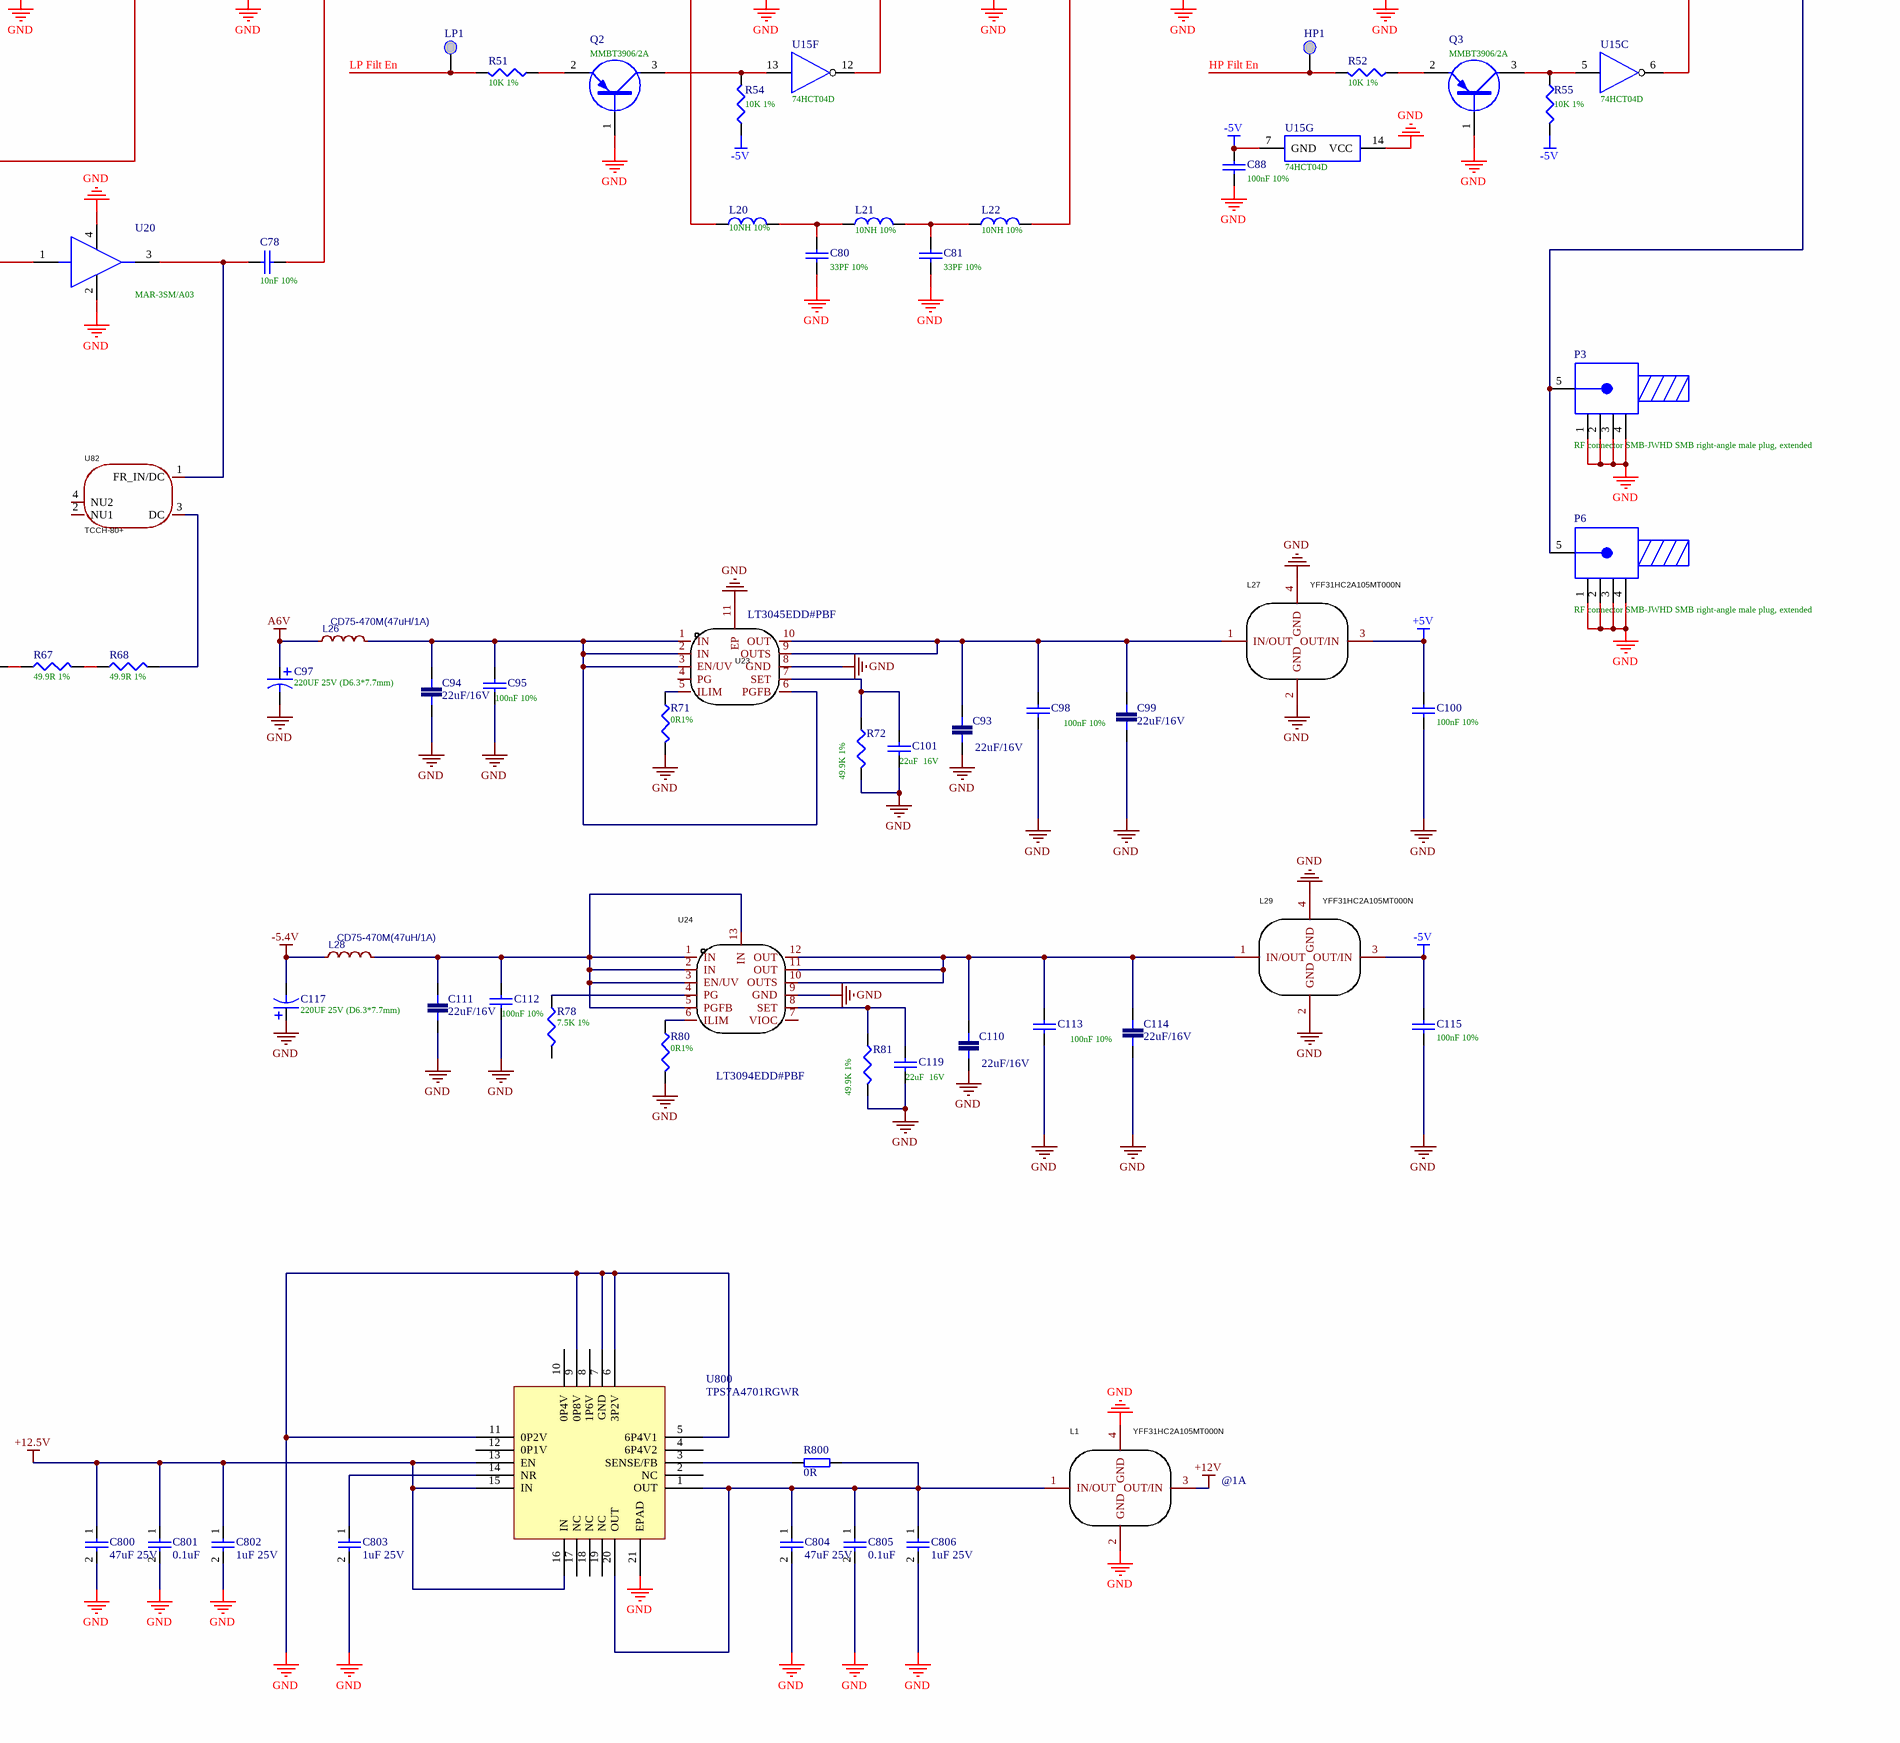
[diagram p0: PCBE109560-7.SchDoc, bottom right]
# Altium schematic sheet PCBE109560-7.SchDoc (part 2 of 2)

## Parts
1  (no value)  [DIP-1]
+1  (no value)  [DIP-1]
+2  (no value)  [DIP-1]
C4  20PF 10%  [0805C]
C5  330PF 10%  [1812C]
C6  22PF 10%  [1812C-2]
C7  22uF/16V  [0805]
C8  22uF/16V  [0805]
C9  100nF 10%  [0603]
C10  220UF 25V (D6.3*7.7mm)  [CAP-SMD_BD6.3-L6.6-W6.6-FD]
C11  100nF 10%  [0603]
C12  22uF/16V  [0805]
C13  100nF 10%  [0805R]
C14  22uF  16V  [0805]
C15  100nF 10%  [0805R]
C16  47PF 10%  [1812C-2]
C17  100PF 10%  [1812C-2]
C18  20PF 10%  [0805R]
C20  100nF 10%  [0805R]
C21  100nF 10%  [0805R]
C31  100nF 10%  [0805R]
C32  100nF 10%  [0805R]
C34  100nF 10%  [0805R]
C35  100nF 10%  [0805R]
C36  100nF 10%  [0805R]
C37  100nF 10%  [0805R]
C39  100nF 10%  [0805R]
C40  100nF 10%  [0805R]
C41  100nF 10%  [0805R]
C42  100nF 10%  [0805R]
C43  100nF 10%  [0805R]
C44  100nF 10%  [0805R]
C45  100nF 10%  [0805R]
C46  100nF 10%  [0805R]
C47  100nF 10%  [0805R]
C48  100nF 10%  [0805R]
C49  22uF 25V  [CAP-SMD_L6.0-W3.2-R-RD]
C50  100nF 10%  [0805R]
C51  100nF 10%  [0805R]
C52  100nF 10%  [0805R]
C53  3.3NF 10%  [0805R]
C54  100nF 10%  [0805R]
C55  330PF 10%  [0805R]
C56  330PF 10%  [0805R]
C57  100nF 10%  [0805R]
C58  33PF 10%  [0805R]
C59  33PF 10%  [0805R]
C60  100nF 10%  [0805R]
C61  100nF 10%  [0805R]
C62  100nF 10%  [0805R]
C63  100nF 10%  [0805R]
C64  100nF 10%  [0805R]
C65  33PF 10%  [0805R]
C66  33PF 10%  [0805R]
C67  100nF 10%  [0805R]
C68  39PF 10%  [0805R]
C69  100nF 10%  [0805R]
C70  25V 1UF Type A  [0805C-2]
C71  25V 1UF Type A  [0805C-2]
C72  100nF 10%  [0805R]
C73  25V 1UF Type A  [0805C-2]
C74  100nF 10%  [0805R]
C75  100nF 10%  [0805R]
C76  10nF 10%  [0805R]
C77  10nF 10%  [0805R]
C78  10nF 10%  [0805R]
C79  100nF 10%  [0603C]
C80  33PF 10%  [0805R]
C81  33PF 10%  [0805R]
C82  100nF 10%  [0805R]
C83  100nF 10%  [0805R]
C84  100nF 10%  [0805R]
C85  100nF 10%  [0805R]
C86  25V 1UF Type A  [0805C-2]
C87  3pF( ±0.1pF)  [0805R]
C88  100nF 10%  [0805R]
C89  100nF 10%  [0805R]
C90  100nF 10%  [0805R]
C93  22uF/16V  [0805]
C94  22uF/16V  [0805]
C95  100nF 10%  [0603]
C96  100nF 10%  [0805R]
C97  220UF 25V (D6.3*7.7mm)  [CAP-SMD_BD6.3-L6.6-W6.6-FD]
C98  100nF 10%  [0603]
C99  22uF/16V  [0805]
C100  100nF 10%  [0805R]
C101  22uF  16V  [0805]
C102  100nF 10%  [0805R]
C103  100nF 10%  [0805R]
C104  100nF 10%  [0805R]
C105  100nF 10%  [0805R]
C106  100nF 10%  [0805R]
C107  100nF 10%  [0805R]
C109  100nF 10%  [0805R]
C110  22uF/16V  [0805]
C111  22uF/16V  [0805]
C112  100nF 10%  [0603]
C113  100nF 10%  [0603]
C114  22uF/16V  [0805]
C115  100nF 10%  [0805R]
C116  100nF 10%  [0805R]
C117  220UF 25V (D6.3*7.7mm)  [CAP-SMD_BD6.3-L6.6-W6.6-FD]
C118  100nF 10%  [0805R]
C119  22uF  16V  [0805]
C122  100nF 10%  [0805R]
C123  100nF 10%  [0805R]
C124  100nF 10%  [0805R]
C125  100nF 10%  [0805R]
C128  100nF 10%  [0805R]
C129  100nF 10%  [0805R]
C130  100nF 10%  [0805R]
C800  47uF 25V  [1206]
C801  0.1uF  [0402]
C802  1uF 25V  [0402]
C803  1uF 25V  [0402]
C804  47uF 25V  [1206]
C805  0.1uF  [0402]
C806  1uF 25V  [0402]
C?  100nF 10%  [0805R]
Clk1  (no value)  [DIP-1]
D1  BAV99/A7  [SOT-23]
D2  GF1M-E3/67A/GM  [1808D]
D3  GF1M-E3/67A/GM  [1808D]
D4  GF1M-E3/67A/GM  [1808D]
D5  GF1M-E3/67A/GM  [1808D]
D8  BAV99/A7  [SOT-23-2]
D9  BAV99/A7  [SOT-23-2]
D10  BAV99/A7  [SOT-23-2]
D11  BAV99/A7  [SOT-23-2]
D12  BAV99/A7  [SOT-23-2]
Data1  (no value)  [DIP-1]
HP1  (no value)  [DIP-1]
J1  RF connector  [DIP-P]
J2  RF connector  [DIP-P]
L1  YFF31HC2A105MT000N  [FILTER-SMD_4P-L3.2-W1.6-L_YFF31HC]
L2  15UH 5%  [1005R]
L3  BLM21PG221SN1D(220Ω@100MHz)  [0805R]
L4  YFF31HC2A105MT000N  [FILTER-SMD_4P-L3.2-W1.6-L_YFF31HC]
L5  6.8UH 10%  [0805R]
L8  YFF31HC2A105MT000N  [FILTER-SMD_4P-L3.2-W1.6-L_YFF31HC]
L10  10NH 10%  [0805R]
L11  10NH 10%  [0805R]
L12  10NH 10%  [0805R]
L13  YFF31HC2A105MT000N  [FILTER-SMD_4P-L3.2-W1.6-L_YFF31HC]
L15  4.7UH 5%  [1005L]
L16  1UH 5%  [0805R]
L17  BLM21PG221SN1D(220Ω@100MHz)  [0805R]
L18  BLM21PG221SN1D(220Ω@100MHz  [0805R]
L19  NFM15PC104R1A3D  [FILTER-SMD_0402-3P-L1.0-W0.5-T]
L20  10NH 10%  [0805R]
L21  10NH 10%  [0805R]
L22  10NH 10%  [0805R]
L23  YFF31HC2A105MT000N  [FILTER-SMD_4P-L3.2-W1.6-L_YFF31HC]
L24  YFF31HC2A105MT000N  [FILTER-SMD_4P-L3.2-W1.6-L_YFF31HC]
L25  BLM21PG221SN1D(220Ω@100MHz  [0805R]
L26  CD75-470M(47uH/1A)  [IND-SMD_L7.8-W7.0-A]
L27  YFF31HC2A105MT000N  [FILTER-SMD_4P-L3.2-W1.6-L_YFF31HC]
L28  CD75-470M(47uH/1A)  [IND-SMD_L7.8-W7.0-A]
L29  YFF31HC2A105MT000N  [FILTER-SMD_4P-L3.2-W1.6-L_YFF31HC]
L31  BLM21PG221SN1D(220Ω@100MHz  [0805R]
L32  BLM21PG221SN1D(220Ω@100MHz  [0805R]
L808  NFM15PC104R1A3D  [FILTER-SMD_0402-3P-L1.0-W0.5-T]
L809  NFM15PC104R1A3D  [FILTER-SMD_0402-3P-L1.0-W0.5-T]
L810  NFM15PC104R1A3D  [FILTER-SMD_0402-3P-L1.0-W0.5-T]
L811  NFM15PC104R1A3D  [FILTER-SMD_0402-3P-L1.0-W0.5-T]
L812  NFM15PC104R1A3D  [FILTER-SMD_0402-3P-L1.0-W0.5-T]
L813  NFM15PC104R1A3D  [FILTER-SMD_0402-3P-L1.0-W0.5-T]
LP1  (no value)  [DIP-1]
P1  Header 20X2  [N0.8mm/40Pin-Plug]
P2  Header 4X2  [N0.8mm/8Pin-SOCKET]
P3  RF connector SMB-JWHD SMB right-angle male plug, extended  [DIP-P-2]
P4  Header 20X2  [N0.8mm/40Pin-Plug]
P5  Header 20X2  [N0.8mm/40Pin-Plug]
P6  RF connector SMB-JWHD SMB right-angle male plug, extended  [DIP-P-2]
Q1  MJD31C  [SOT-252-2]
Q2  MMBT3906/2A  [SOT-23]
Q3  MMBT3906/2A  [SOT-23]
Q4  MMBT3906/2A  [SOT-23]
R6  2K 5%  [0603R]
R7  NC  [AXIAL-0.51]
R8  3.9K 5% 1/2W  [AXIAL-0.51]
R9  3.9K 5% 1/2W  [AXIAL-0.51]
R10  3.9K 5% 1/2W  [AXIAL-0.51]
R11  3.9K 5% 1/2W  [AXIAL-0.51]
R13  0R1%  [0603]
R14  49.9K 1%  [0603]
R15  4.99K 1%  [0805R]
R16  2K 1%  [0805R]
R17  49.9R 1% 1/4W  [AXIAL-0.4]
R20  100R 1% 1/4W  [AXIAL-0.4]
R23  100R 1% 1/4W  [AXIAL-0.4]
R27  4.87K 1%  [0805R]
R28  4.87K 1%  [0805R]
R29  4.87K 1%  [0805R]
R30  4.87K 1%  [0805R]
R31  4.87K 1%  [0805R]
R32  10K 1%  [0805R]
R33  100K 1%  [0805R]
R34  100K 1%  [0805R]
R35  49.9R 1%  [0805R]
R36  49.9R 1%  [0805R]
R37  49.9R 1%  [0805R]
R38  49.9R 1%  [0805R]
R39  49.9R 1%  [0805R]
R40  49.9R 1% 1/4W  [R-SMD_L3.5-W1.5]
R41  10K 1%  [0805R]
R42  4.87K 1%  [0805R]
R43  4.87K 1%  [0805R]
R44  4.87K 1%  [0805R]
R45  4.87K 1%  [0805R]
R46  169R 1%  [0805R]
R47  169R 1%  [0805R]
R48  169R 1%  [0805R]
R49  49.9R 1%  [0805R]
R50  49.9R 1%  [0805R]
R51  10K 1%  [0805R]
R52  10K 1%  [0805R]
R53  10K 1%  [0805R]
R54  10K 1%  [0805R]
R55  10K 1%  [0805R]
R56  10K 1%  [0805R]
R57  10K 1%  [0805R]
R58  49.9R 1%  [0805R]
R59  4.99K 1%  [0805R]
R60  49.9R 1%  [R-SMD_L3.5-W1.5]
R61  30R 1%  [R-SMD_L3.5-W1.5]
R62  169R 1%  [0805R]
R63  169R 1%  [0805R]
R64  169R 1%  [0805R]
R65  49.9R 1%  [0805R]
R66  49.9R 1%  [0805R]
R67  49.9R 1%  [0805R]
R68  49.9R 1%  [0805R]
R69  120R 1%  [R-SMD_L3.5-W1.5]
R70  169R 1%  [0805R]
R71  0R1%  [0603]
R72  49.9K 1%  [0603]
R73  169R 1%  [0805R]
R74  NC  [0805R]
R75  169R 1%  [0805R]
R77  169R 1%  [0805R]
R78  7.5K 1%  [0603]
R80  0R1%  [0603]
R81  49.9K 1%  [0603]
R82  100K 1%  [0805R]
R83  10K 1%  [0805R]
R84  169R 1%  [0805R]
R800  0R  [0402]
RE1  AGQ210A4HZ  [RELAY-SMD_PANASONIC_AGQ2X0AXX]
RE2  AGQ210A4HZ  [RELAY-SMD_PANASONIC_AGQ2X0AXX]
RE3  AGQ210A4HZ  [RELAY-SMD_PANASONIC_AGQ2X0AXX]
RE4  AGQ210A4HZ  [RELAY-SMD_PANASONIC_AGQ2X0AXX]
RE5  AGQ210A4HZ  [RELAY-SMD_PANASONIC_AGQ2X0AXX]
Strobe1  (no value)  [DIP-1]
U4  LT3045EDD#PBF  [DFN-10_L3.0-W3.0-P0.50-BL-EP]
U6  74HCT123D  [SOIC-16_L9.9-W3.9-P1.27-LS6.0-BL]
U8  MAX504CSD+T  [SO-14]
U9  SW-239  [SO-8]
U11  SW-239  [SO-8]
U12  SW-239  [SO-8]
U13  SW-239  [SO-8]
U14  SW-239  [SO-8]
U15  74HCT04D  [SO-14]  (parts A,B,C,D,E,F,G of 7)
U16  AT-250(MAAV-007941)  [SO-8]
U17  MAR-3SM/A03  [LCC4]
U18  MAR-6SM/A06  [LCC4]
U19  MAR-6SM/A06  [LCC4]
U20  MAR-3SM/A03  [LCC4]
U21  MAX4106ESA+T  [SO-8]
U22  MIC4420CM  [SO-8]
U23  LT3045EDD#PBF  [DFN-10_L3.0-W3.0-P0.50-BL-EP]
U24  LT3094EDD#PBF  [WDFN-12_L3.0-W3.0-P0.45-BL-EP]
U25  AT65-0263  [SO-16]
U80  TCCH-80+  [IND-SMD_4P-L3.8-W3.8]
U81  TCCH-80+  [IND-SMD_4P-L3.8-W3.8]
U82  TCCH-80+  [IND-SMD_4P-L3.8-W3.8]
U83  TCCH-80+  [IND-SMD_4P-L3.8-W3.8]
U100  SW-239  [SO-8]
U800  TPS7A4701RGWR  [QFN-20]

## Nets
+5V: C100.1 C?.1 L25.1 L27.3(OUT/IN) L811.3(OUTPUT) L812.3(OUTPUT) U8.3(~{CLR})
+12.5V: +2.1 C106.1 C800.1 C801.1 C802.1 P5.31 P5.32 P5.33 P5.34 P5.35 P5.36 P5.37 P5.38 P5.39 P5.40 U800.13(EN) U800.15(IN) U800.16(IN)
+12V: C122.1 C123.1 C124.2 C125.2 L1.3(OUT/IN) L8.1(IN/OUT) L13.1(IN/OUT) U22.1(VS) U22.8(VS)
-5.4V: +1.1 C107.1 C117.2 L28.2 P5.1 P5.2 P5.3 P5.4 P5.5 P5.6 P5.7 P5.8 P5.9 P5.10
-5V: C88.2 C115.2 L29.3(OUT/IN) L809.1(INPUT) L810.3(OUTPUT) L813.3(OUTPUT) R54.1 R55.2 R57.1 U15.7(GND)
A6V: 1.1 C10.1 C97.1 C103.2 L3.1 L26.2 P5.17 P5.18 P5.19 P5.20 P5.21 P5.22 P5.23 P5.24
GND: C5.1 C6.2 C7.1 C8.1 C9.2 C10.2 C11.2 C12.1 C13.2 C14.2 C15.1 C18.2 C20.1 C21.1 C31.1 C32.1 C34.1 C35.1 C36.2 C37.2 C39.2 C40.2 C42.2 C43.1 C44.2 C45.2 C46.2 C47.1 C48.1 C49.2 C50.2 C57.2 C60.2 C61.1 C62.1 C63.1 C64.1 C65.2 C66.1 C70.1 C71.1 C72.2 C73.1 C74.1 C75.1 C80.1 C81.1 C83.2 C84.2 C85.1 C86.2 C88.1 C89.2 C90.2 C93.1 C94.1 C95.2 C96.2 C97.2 C98.2 C99.1 C100.2 C101.2 C102.2 C103.1 C104.2 C105.1 C106.2 C107.2 C109.2 C110.1 C111.1 C112.2 C113.2 C114.1 C115.1 C117.1 C118.2 C119.2 C122.2 C123.2 C124.1 C125.1 C128.1 C129.1 C130.2 C800.2 C801.2 C802.2 C803.2 C804.2 C805.2 C806.2 C?.2 D1.3 D2.2(K) D11.2 D12.1 J1.1 J1.2 J1.3 J1.4 J2.1 J2.2 J2.3 J2.4 L1.2(GND) L1.4(GND) L2.2 L4.2(GND) L4.4(GND) L8.2(GND) L8.4(GND) L13.2(GND) L13.4(GND) L15.2 L16.1 L19.2(GND) L23.2(GND) L23.4(GND) L24.2(GND) L24.4(GND) L27.2(GND) L27.4(GND) L29.2(GND) L29.4(GND) L808.2(GND) L809.2(GND) L810.2(GND) L811.2(GND) L812.2(GND) L813.2(GND) P1.5 P1.6 P1.11 P1.12 P1.17 P1.18 P1.20 P1.23 P1.24 P1.29 P1.30 P1.35 P1.36 P2.1 P2.3 P2.5 P2.7 P3.1 P3.2 P3.3 P3.4 P4.5 P4.6 P4.11 P4.12 P4.17 P4.18 P4.23 P4.24 P4.29 P4.30 P4.35 P4.36 P5.11 P5.12 P5.13 P5.14 P5.15 P5.16 P5.25 P5.26 P5.27 P5.28 P5.29 P5.30 P6.1 P6.2 P6.3 P6.4 Q1.2(E) Q2.1(B) Q3.1(B) Q4.1(B) R13.2 R14.2 R20.2 R32.2 R53.1 R59.1 R61.1 R71.2 R72.2 R74.1 R80.2 R81.2 R82.1 R83.1 RE1.3 RE3.6 RE4.2 U4.8(GND) U4.11(EP) U6.6(2CEXT) U6.8(GND) U6.10(2B) U6.14(1CEXT) U8.7(DGND) U8.8(AGND) U9.2(GND) U9.7(GND) U9.8(GND) U11.2(GND) U11.7(GND) U11.8(GND) U12.2(GND) U12.7(GND) U12.8(GND) U13.2(GND) U13.7(GND) U13.8(GND) U14.2(GND) U14.7(GND) U14.8(GND) U15.14(VCC) U16.2(GND) U16.3(GND) U16.5(GND) U16.6(GND) U16.7(GND) U17.2(GND) U17.4(GND) U18.2(GND) U18.4(GND) U19.2(GND) U19.4(GND) U20.2(GND) U20.4(GND) U22.4(GND) U22.5(GND) U23.8(GND) U23.11(EP) U24.9(GND) U25.2(GND) U25.3(GND) U25.4(GND) U25.5(GND) U25.6(GND) U25.7(GND) U25.16(GND) U100.2(GND) U100.7(GND) U100.8(GND) U800.5(6P4V1) U800.6(3P2V) U800.7(GND) U800.9(0P8V) U800.11(0P2V) U800.21(EPAD)
VCC: C13.1 C15.2 L4.3(OUT/IN) R15.1 R16.2 U6.2(1B) U6.3(1~{R}D) U6.16(VCC)
AK2: C21.2 P1.33 RE1.1
AK3: C20.2 P1.38 RE1.8
AK4: C37.1 P1.37 RE2.1
AK5: C36.1 P1.40 RE2.8
AK6: C31.2 P1.34 RE3.8
AK7: C32.2 P1.32 RE3.1
AK8: C34.2 C40.1 P1.28 RE4.8 RE5.8
AK9: C35.2 C39.1 P1.26 RE4.1 RE5.1
Attn1: P4.34 R70.2
Attn2: P4.32 R73.2
Attn4: P4.28 R75.2
Attn8: P4.26 R77.2
Attn16: P4.22 R84.2
DAC Clk: Clk1.1 P4.14 U8.4(SCLK)
DAC Data: Data1.1 P4.16 U8.2(DIN)
DAC Strobe: P4.10 Strobe1.1 U8.5(~{CS})
DATA_T: P1.39 R15.2 U6.1(1~{A})
HP Filt En: HP1.1 P4.4 R52.2
HT: L5.1 P2.2 P2.4 P2.6 P2.8
IN2: P4.8 R56.1 U22.2(IN)
LP Filt En: LP1.1 P4.2 R51.2
NetC4_1: C4.1 D1.2 L2.1 Q1.1(B) R6.1
NetC4_2: C4.2 R6.2 U6.13(1Q)
NetC5_2: C5.2 L5.2 R7.2
NetC6_1: C6.1 C16.2 C17.2 Q1.3(C) R11.1
NetC7_2: C7.2 C11.1 C12.2 L4.1(IN/OUT) U4.9(OUTS) U4.10(OUT)
NetC8_2: C8.2 C9.1 L3.2 U4.1(IN) U4.2(IN) U4.3(EN/UV) U4.6(PGFB)
NetC14_1: C14.1 R14.1 U4.7(SET)
NetC16_1: C16.1 D5.1(A) D8.2 D9.2 RE2.6
NetC17_1: C17.1 RE2.7
NetC18_1: C18.1 R16.1 U6.15(1REXT/CEXT)
NetC41_1: C41.1 U14.1(RFCOM)
NetC41_2: C41.2 P3.5 P6.5 R32.1
NetC42_1: C42.1 R27.1 U9.5(B)
NetC43_2: C43.2 R28.2 U100.4(A)
NetC44_1: C44.1 R29.1 U11.4(A)
NetC45_1: C45.1 R30.1 U12.5(B)
NetC46_1: C46.1 R31.1 U13.5(B) U14.4(A)
NetC47_2: C47.2 R35.1 U16.4(A)
NetC48_2: C48.2 L8.3(OUT/IN) R36.1
NetC49_1: C49.1 C50.1 U8.1(BIPOFF) U8.9(REFIN) U8.10(REFOUT)
NetC51_1: C51.1 U17.1(RF_IN)
NetC51_2: C51.2 U16.8(RF2)
NetC52_1: C52.1 L10.2
NetC52_2: C52.2 U17.3(RF_OUT) U81.1(FR_IN/DC)
NetC53_1: C53.1 C54.1 L15.1
NetC53_2: C53.2 U12.1(RFCOM)
NetC54_2: C54.2 U13.1(RFCOM)
NetC55_1: C55.1 U13.3(RF1)
NetC55_2: C55.2 C56.1 L16.2
NetC56_2: C56.2 U14.6(RF2)
NetC57_1: C57.1 R41.1 U13.4(A) U14.5(B)
NetC58_1: C58.1 C65.1
NetC58_2: C58.2 L10.1 L11.1
NetC59_1: C59.1 L11.2 L12.1
NetC59_2: C59.2 C66.2
NetC60_1: C60.1 R42.1 U9.4(A)
NetC61_2: C61.2 R43.2 U100.5(B)
NetC62_2: C62.2 R44.1 U11.5(B)
NetC63_2: C63.2 R45.1 U12.4(A)
NetC64_2: C64.2 L13.3(OUT/IN) R46.2
NetC67_1: C67.1 U18.1(RF_IN)
NetC67_2: C67.2 U25.1(RF)
NetC68_1: C68.1 C69.2 R49.2 R50.2
NetC68_2: C68.2 R49.1 R50.1 U18.3(RF_OUT) U80.1(FR_IN/DC)
NetC69_1: C69.1 R53.2 U16.1(RF1)
NetC70_2: C70.2 C74.2 L18.1 L19.1(INPUT)
NetC71_2: C71.2 C75.2 L19.3(OUTPUT) U21.4(VEE)
NetC72_1: C72.1 C73.2 L17.2 L18.2
NetC76_1: C76.1 U9.3(RF1)
NetC76_2: C76.2 U19.1(RF_IN)
NetC77_1: C77.1 U19.3(RF_OUT) U83.1(FR_IN/DC)
NetC77_2: C77.2 U20.1(RF_IN)
NetC78_1: C78.1 U20.3(RF_OUT) U82.1(FR_IN/DC)
NetC78_2: C78.2 U100.6(RF2)
NetC79_1: C79.1 D10.3 R40.2
NetC79_2: C79.2 R58.2 R59.2
NetC80_2: C80.2 L20.2 L21.2
NetC81_2: C81.2 L21.1 L22.1
NetC82_1: C82.1 R60.2
NetC82_2: C82.2 C116.1 R74.2 R82.2
NetC83_1: C83.1 C86.1 L808.1(INPUT) U21.7(VCC)
NetC84_1: C84.1 L23.3(OUT/IN) R62.2
NetC85_2: C85.2 L24.3(OUT/IN) R65.1
NetC87_1: C87.1 R60.1 R69.1 U21.6(OUT)
NetC87_2: C87.2 R61.2 R69.2 U21.2(IN-)
NetC89_1: C89.1 L813.1(INPUT) U8.11(VSS)
NetC90_1: C90.1 L32.2 L811.1(INPUT)
NetC93_2: C93.2 C98.1 C99.2 L27.1(IN/OUT) U23.9(OUTS) U23.10(OUT)
NetC94_2: C94.2 C95.1 L26.1 U23.1(IN) U23.2(IN) U23.3(EN/UV) U23.6(PGFB)
NetC96_1: C96.1 R70.1 U25.15(C1)
NetC101_1: C101.1 R72.1 U23.7(SET)
NetC102_1: C102.1 R73.1 U25.14(C2)
NetC104_1: C104.1 L812.1(INPUT) U8.13(VDD)
NetC105_2: C105.2 L31.1 L810.1(INPUT)
NetC109_1: C109.1 R75.1 U25.13(C4)
NetC110_2: C110.2 C113.1 C114.2 L29.1(IN/OUT) U24.10(OUTS) U24.11(OUT) U24.12(OUT)
NetC111_2: C111.2 C112.1 L28.1 U24.1(IN) U24.2(IN) U24.3(EN/UV) U24.5(PGFB) U24.13(IN)
NetC116_2: C116.2 R83.2 U25.8(RF)
NetC118_1: C118.1 R77.1 U25.12(C8)
NetC119_1: C119.1 R81.1 U24.8(SET)
NetC128_2: C128.2 L31.2 U25.11(VEE)
NetC129_2: C129.2 L32.1 U25.10(VCC)
NetC130_1: C130.1 R84.1 U25.9(C16)
NetC803_1: C803.1 U800.14(NR)
NetC804_1: C804.1 C805.1 C806.1 L1.1(IN/OUT) R800.1 U800.1(OUT) U800.20(OUT)
NetD2_1: D2.1(A) D3.2(K)
NetD3_1: D3.1(A) D4.2(K)
NetD4_1: D4.1(A) D5.2(K)
NetD8_1: D8.1 D9.1 J1.5 R17.1 R20.1 R23.1 RE4.4
NetD10_1: D10.1 D12.2
NetD10_2: D10.2 D11.1
NetJ2_5: J2.5 RE5.4
NetL12_2: L12.2 U9.1(RFCOM)
NetL17_1: L17.1 L809.3(OUTPUT)
NetL20_1: L20.1 U11.6(RF2)
NetL22_2: L22.2 U12.3(RF1)
NetL23_1: L23.1(IN/OUT) L24.1(IN/OUT) U22.6(OUT) U22.7(OUT)
NetL25_2: L25.2 L808.3(OUTPUT)
NetQ2_2: Q2.2(E) R51.1
NetQ2_3: Q2.3(C) R54.2 U15.13(6A)
NetQ3_2: Q3.2(E) R52.1
NetQ3_3: Q3.3(C) R55.1 U15.5(3A)
NetQ4_2: Q4.2(E) R56.2
NetQ4_3: Q4.3(C) R57.2 U15.1(1A)
NetR7_1: R7.1 R8.1
NetR8_2: R8.2 R9.2
NetR9_1: R9.1 R10.1
NetR10_2: R10.2 R11.2
NetR13_1: R13.1 U4.5(ILIM)
NetR17_2: R17.2 RE1.2
NetR23_2: R23.2 RE3.7
NetR27_2: R27.2 R28.1 U15.4(2Y)
NetR29_2: R29.2 R30.2 U15.10(5Y)
NetR31_2: R31.2 U15.8(4Y)
NetR33_1: R33.1 R34.1 U8.14(RFB)
NetR33_2: R33.2 R34.2 R35.2 U8.12(VOUT)
NetR36_2: R36.2 R37.1
NetR37_2: R37.2 R38.2
NetR38_1: R38.1 R39.1
NetR39_2: R39.2 U81.3(DC)
NetR40_1: R40.1 RE5.3
NetR41_2: R41.2 U15.6(3Y) U15.9(4A)
NetR42_2: R42.2 R43.1 U15.2(1Y) U15.3(2A)
NetR44_2: R44.2 R45.2 U15.11(5A) U15.12(6Y)
NetR46_1: R46.1 R47.2
NetR47_1: R47.1 R48.1
NetR48_2: R48.2 U80.3(DC)
NetR58_1: R58.1 U21.3(IN+)
NetR62_1: R62.1 R63.1
NetR63_2: R63.2 R64.2
NetR64_1: R64.1 U83.3(DC)
NetR65_2: R65.2 R66.2
NetR66_1: R66.1 R67.1
NetR67_2: R67.2 R68.1
NetR68_2: R68.2 U82.3(DC)
NetR71_1: R71.1 U23.5(ILIM)
NetR78_1: R78.1 U24.4(PG)
NetR80_1: R80.1 U24.6(ILIM)
NetR800_2: R800.2 U800.3(SENSE/FB)
NetRE4_3: RE4.3 RE5.2
NetU9_6: U9.6(RF2) U100.3(RF1)
NetU11_1: U11.1(RFCOM) U100.1(RFCOM)
NetU11_3: U11.3(RF1) U12.6(RF2)
NetU13_6: U13.6(RF2) U14.3(RF1)

Not connected (* = marked no-connect by the designer): D1 1*; D8 3; D9 3; D11 3; D12 3; P1 1 2 3 4 7 8 9 10 13 14 15 16 19 21 22 25 27 31; P4 1 3 7 9 13 15 19 20 21 25 27 31 33 37 38 39 40; R78 2; RE1 4 5 6 7; RE2 2 3 4 5; RE3 2 3 4 5; RE4 5 6 7; RE5 5 6 7; U4 4(PG); U6 4(1~{Q}) 5(2Q) 7(2REXT/CEXT) 9(2~{A}) 11(2~{R}D) 12(2~{Q}); U8 6(DOUT); U22 3(NC); U23 4(PG); U24 7(VIOC); U80 2(NU1) 4(NU2); U81 2(NU1) 4(NU2); U82 2(NU1) 4(NU2); U83 2(NU1) 4(NU2); U800 2(NC) 4(6P4V2) 8(1P6V) 10(0P4V) 12(0P1V) 17(NC) 18(NC) 19(NC)

## Notes on the sheet
- (near P1) Transmit interface
- 500V high-voltage interface
- Receive interface
- @1A

## Library data of the parts
1 +1 +2 Clk1 Data1 HP1 LP1 Strobe1 = TP
C4-C6 C9 C11 C13-C18 C20 C21 C31 C32 C34-C37 C39-C48 C50-C69 C72-C85 C87-C90 C95 C96 C98 C100-C107 C109 C112 C113 C115 C116 C118 C119 C122-C125 C128-C130 C800-C806 C? = CAP: Capacitor
C7 C8 C12 C93 C94 C99 C110 C111 C114 = C1206
C10 C97 C117 = CAPACITOR_1: Capacitor
C49 = TAJC226K025RNJ: Manufacturer: Kyocera AVX; Add into BOM: yes; Tolerance: ±10%; Equivalent Series Resistance(ESR): 1.4Ω@100kHz; Symbol: TAJC226K025RNJ; Device: TAJC226K025RNJ; LCSC Part Name: 22uF ±10% 25V; Supplier Part: C7214; Manufacturer Part: TAJC226K025RNJ; Supplier Footprint: CASE-C-6032; JLCPCB Part Class: Extended Part; Datasheet: https://atta.szlcsc.com/upload/public/pdf/source/20160107/1457707750344.pdf; Supplier: LCSC; Convert to PCB: yes; Value: 22uF; Rated Voltage: 25V; Operating Temperature: -55℃~+125℃
C70 C71 C86 = CAPACITOR POL: Capacitor
D1 D8-D12 = BAV99
D2-D5 = DIODE
J1 J2 = SMA-KWE: BOM_Supplier: *; BOM_Supplier Part: *; BOM_Manufacturer: *; BOM_Manufacturer Part: *; BOM_JLCPCB Part Class: *; spicePre: *; spiceSymbolName: *; Contributor: *
L1 L4 L8 L13 L23 L24 L27 L29 = YFF31HC2A105MT000N: Manufacturer: TDK; Add into BOM: yes; Nominal Capacitance: 1uF; CapacitanceTolerance: ±20%; DC Rated Voltage: 100V; Rated Current: 6A; DC Resistance: 5mΩ; Name: YFF31HC2A105MT000N; Symbol: YFF31HC2A105MT000N; Device: YFF31HC2A105MT000N; LCSC Part Name: 1uF(105) ±20% 100V; Supplier Part: C113216; Manufacturer Part: YFF31HC2A105MT000N; Supplier Footprint: SMD-4P,1.6x3.2mm; JLCPCB Part Class: Extended Part; Datasheet: https://atta.szlcsc.com/upload/public/pdf/source/20180326/C113216_F6F81E50B9805DA3D7C436129903DEBD.pdf; Supplier: LCSC; Convert to PCB: yes; Operating Temperature: -55℃~+125℃
L2 L3 L5 L10-L12 L15-L18 L20-L22 L25 L31 L32 = INDUCTOR
L19 L808-L813 = NFM15PC104R1A3D: Manufacturer: muRata(村田); Add into BOM: yes; Nominal Capacitance: 100nF; CapacitanceTolerance: ±20%; DC Rated Voltage: 10V; Rated Current: 2A; DC Resistance: 30mΩ; Symbol: NFM15PC104R1A3D; Device: NFM15PC104R1A3D; LCSC Part Name: 0.1uF ±20% 10V; Supplier Part: C2650905; Manufacturer Part: NFM15PC104R1A3D; Supplier Footprint: 0402; JLCPCB Part Class: Extended Part; Datasheet: https://atta.szlcsc.com/upload/public/pdf/source/20210611/05FD8D968916F804F398094FB2B4AAFE.pdf; Supplier: LCSC; Convert to PCB: yes; Operating Temperature: -55℃~+105℃; Comment_1: NFM15PC104R1A3D
L26 L28 = 4.7uH/5a: BOM_Manufacturer: COILMX; BOM_Manufacturer Part: MS0630-4R7M; nameAlias: Inductance; Contributor: LCSC; BOM_Supplier: LCSC; BOM_Supplier Part: C380177; spicePre: L; spiceSymbolName: MS0630-4R7M
P1 P4 P5 = Header 20X2: Header, 20-Pin, Dual row; LatestRevisionDate: 17-Jul-2002; LatestRevisionNote: Re-released for DXP Platform.; Publisher: Altium Limited
P2 = Header 4X2: Header, 4-Pin, Dual row; LatestRevisionDate: 17-Jul-2002; LatestRevisionNote: Re-released for DXP Platform.; Publisher: Altium Limited
P3 P6 = JA1
Q1 = NPN: NPN Transistor
Q2-Q4 = PNP: PNP Transistor
R6-R11 R13-R17 R20 R23 R27-R75 R77 R78 R80-R84 = RES1
R800 = RES
RE1-RE5 = AGQ210A4HZ: Manufacturer: PANASONIC(松下); Add into BOM: yes; Coil Voltage: 4.5V; Contact Form: Two changeover sets: 2C (DPDT changeover); Maximum Switching Voltage: 125V@AC; 110V@DC; Coil Type: Single coil; Maximum Switching Current: 2A; Operate Time: 4ms; Symbol: AGQ210A4HZ; Device: AGQ210A4HZ; LCSC Part Name: AGQ210A4HZ; Supplier Part: C2153577; Manufacturer Part: AGQ210A4HZ; Supplier Footprint: SMD,7.2x10.6mm; JLCPCB Part Class: Extended Part; Datasheet: https://atta.szlcsc.com/upload/public/pdf/source/20210727/C2858037_82AE1FE69E1888D41D6E9B5D42950540.pdf; Supplier: LCSC; Convert to PCB: yes; Pin Number: -; Contact Rating: -; Contact Material: AgPd + gold plating; Coil Rated Power: -; Coil Resistance: -; Release Time: 4ms; Contact Resistance: -; Operating Temperature: -40℃~+85℃; Comment_1: AGQ210A4HZ
U4 U23 = LT3045EDD#PBF: Symbol: LT3045EDD#PBF_C666574; Add into BOM: yes; Maximum Input Voltage: 20V; Output Voltage: 0V~15V; MAX Output Current: 500mA; Dropout Voltage: 450mV@(500mA); standby current: 20uA; Number of Outputs: 1; Device: LT3045EDD#PBF; LCSC Part Name: LT3045EDD#PBF; Supplier Part: C666574; Manufacturer Part: LT3045EDD#PBF; Supplier Footprint: DFN-10-EP(3x3); JLCPCB Part Class: Extended Part; Datasheet: https://atta.szlcsc.com/upload/public/pdf/source/20200416/C514420_E440C492D6C74EAE6AB301243586F696.pdf; Supplier: LCSC; Convert to PCB: yes
U15 = 74HC04
U16 = AT-250
U17 U20 = MAR-3SM
U18 U19 = MAR-6SM
U21 = MAX4107ESA: Manufacturer: *; Manufacturer Part: *; Supplier Part: *; Supplier: *; link: *; spicePre: *; spiceSymbolName: *; Package Display: *; Contributor: *
U24 = LT3094EDD#PBF: Add into BOM: yes; Symbol: LT3094EDD#PBF; Device: LT3094EDD#PBF; LCSC Part Name: LT3094EDD#PBF; Supplier Part: C670492; Manufacturer Part: LT3094EDD#PBF; Supplier Footprint: WDFN-12-EP(3x3); JLCPCB Part Class: Extended Part; Datasheet: https://atta.szlcsc.com/upload/public/pdf/source/20200318/C498217_A5485280C797CF3891C55BEBE66C21D4.pdf; Supplier: LCSC; Convert to PCB: yes; Output Type: -
U80-U83 = TCCH-80+: Manufacturer: Mini-Circuits; Add into BOM: yes; Value: 4uH; Rated Current: 200mA; DC Resistance (DCR): 100mΩ; Symbol: TCCH-80+; Device: TCCH-80+; LCSC Part Name: 4uH; Supplier Part: C3223029; Manufacturer Part: TCCH-80+; Supplier Footprint: SMD-4P,3.8x3.8mm; JLCPCB Part Class: Extended Part; Datasheet: https://atta.szlcsc.com/upload/public/pdf/source/20240402/75EC49D4FFFA61CBEC009CC2CCA83C83.pdf; Supplier: LCSC; Convert to PCB: yes; Tolerance: -; Saturation Current (Isat): -; Type: -; Ratings: -
U800 = TPS7A4701RGWR(QFN20): Name: *; Symbol: *; Device: *; LCSC Part Name: *; Supplier Part: *; Manufacturer: *; Manufacturer Part: *; Supplier Footprint: *; JLCPCB Part Class: *; Datasheet: *; Supplier: *; Add into BOM: *; Convert to PCB: *; Output Type: *; Output Polarity: *; Number of Outputs: *